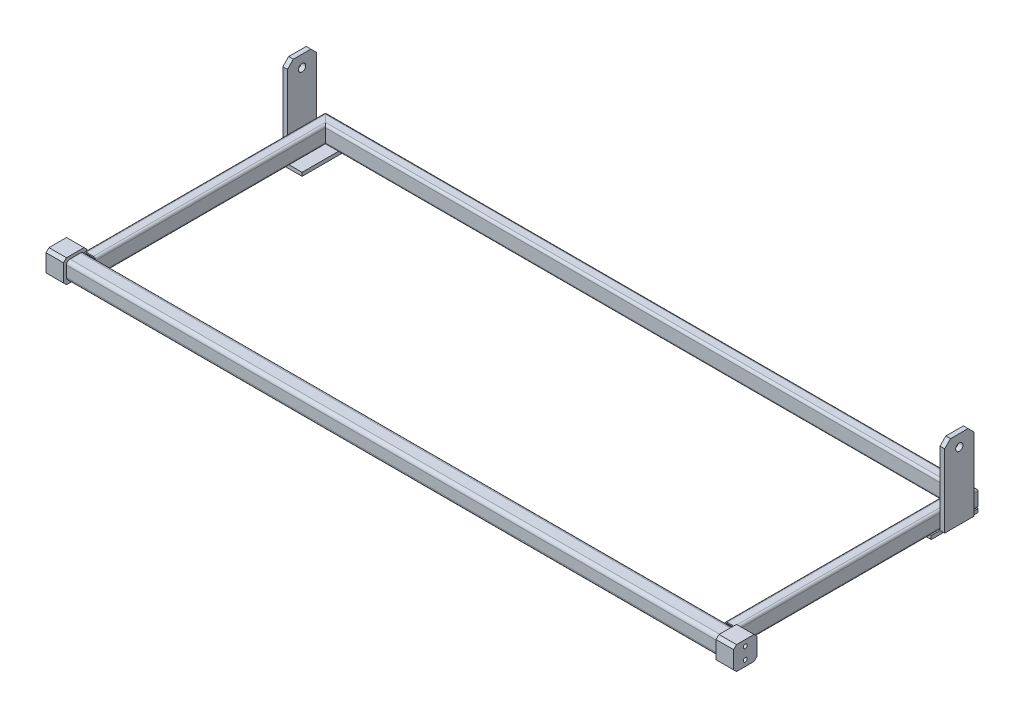
SolidWorks part; units mm, degrees
ref_plane "Front Plane" through (0, 0, 0) normal (0, 0, 1) x (1, 0, 0)
ref_plane "Top Plane" through (0, 0, 0) normal (0, 1, 0) x (1, 0, 0)
ref_plane "Right Plane" through (0, 0, 0) normal (1, 0, 0) x (0, 0, -1)
sketch3d "3DSketch2"
  line L0 (0, 0, 0) -> (1116, 0, 0)
  dimension "D1" = 1116
other "Cold-formed hollow square steel (GB/T 6728-2002) 30×3(1)"
ref_plane "Plane1" through (0, 0, 0) normal (1, 0, 0) x (0, 0, -1)
sketch "Sketch11" plane through (0, 0, 0) normal (1, 0, 0) x (0, 0, -1)
  line L0 (-9, -12) -> (9, -12)
  line L1 (-12, -9) -> (-12, 9)
  line L2 (9, 12) -> (-9, 12)
  line L3 (12, 9) -> (12, -9)
  line L4 (-9, -15) -> (9, -15)
  line L5 (-15, -9) -> (-15, 9)
  line L6 (9, 15) -> (-9, 15)
  line L7 (15, 9) -> (15, -9)
  arc A0 (15, 9) -> (9, 15) centre (9, 9) ccw
  arc A1 (9, -15) -> (15, -9) centre (9, -9) ccw
  arc A2 (-15, -9) -> (-9, -15) centre (-9, -9) ccw
  arc A3 (-9, 15) -> (-15, 9) centre (-9, 9) ccw
  arc A4 (-9, 12) -> (-12, 9) centre (-9, 9) ccw
  arc A5 (12, 9) -> (9, 12) centre (9, 9) ccw
  arc A6 (9, -12) -> (12, -9) centre (9, -9) ccw
  arc A7 (-12, -9) -> (-9, -12) centre (-9, -9) ccw
  point P0 (-15, 0)
  point P1 (15, 0)
  point P2 (0, 15)
  point P3 (0, -15)
  point P4 (0, 0)
  point P5 (-15, -15)
  point P6 (15, -15)
  point P7 (15, 15)
  point P8 (-15, 15)
  point P33 (0, 0)
  dimension "D1" = 6
  dimension "D2" = 30
  dimension "D3" = 3
sketch3d "3DSketch3"
  line L0 (1106, 0, -15) -> (1106, 0, -418)
  line L2 (10, 0, -15) -> (10, 0, -418)
  line L3 (10, 0, -15) -> (1106, 0, -15) construction
  line L4 (10, 0, -418) -> (1106, 0, -418)
  dimension "D1" = 10
  dimension "D2" = 10
  dimension "D3" = 403
other "Cold-formed hollow rectangular steel (GB/T 6728-2002) 30×20×2(1)"
ref_plane "Plane2" through (1106, 0, -15) normal (0, 0, -1) x (1, 0, 0)
sketch "Sketch1" plane through (1106, 0, -15) normal (0, 0, -1) x (1, 0, 0)
  line L0 (-6, -13) -> (6, -13)
  line L1 (-8, -11) -> (-8, 11)
  line L2 (6, 13) -> (-6, 13)
  line L3 (8, 11) -> (8, -11)
  line L4 (-6, -15) -> (6, -15)
  line L5 (-10, -11) -> (-10, 11)
  line L6 (6, 15) -> (-6, 15)
  line L7 (10, 11) -> (10, -11)
  arc A0 (10, 11) -> (6, 15) centre (6, 11) ccw
  arc A1 (6, -15) -> (10, -11) centre (6, -11) ccw
  arc A2 (-10, -11) -> (-6, -15) centre (-6, -11) ccw
  arc A3 (-6, 15) -> (-10, 11) centre (-6, 11) ccw
  arc A4 (-6, 13) -> (-8, 11) centre (-6, 11) ccw
  arc A5 (8, 11) -> (6, 13) centre (6, 11) ccw
  arc A6 (6, -13) -> (8, -11) centre (6, -11) ccw
  arc A7 (-8, -11) -> (-6, -13) centre (-6, -11) ccw
  point P0 (0, 15)
  point P1 (10, 0)
  point P2 (0, -15)
  point P3 (-10, 0)
  point P4 (-10, 15)
  point P5 (10, 15)
  point P6 (10, -15)
  point P7 (-10, -15)
  point P8 (0, 0)
  point P33 (0, 0)
  dimension "D1" = 30
  dimension "D2" = 20
  dimension "D3" = 2
  dimension "D4" = 4
sketch "Sketch4" plane through (0, 0, 0) normal (-1, 0, 0) x (0, 0, 1)
  line L0 (-20, 15) -> (-15, 20)
  line L1 (15, -20) -> (-15, -20)
  line L2 (20, -15) -> (20, 15)
  line L3 (15, 20) -> (-15, 20)
  line L4 (-20, -15) -> (-20, 15)
  line L5 (20, -20) -> (-20, 20) construction
  line L6 (20, 20) -> (-20, -20) construction
  line L7 (20, 15) -> (15, 20)
  line L8 (15, -20) -> (20, -15)
  line L9 (-15, -20) -> (-20, -15)
  point P0 (0, 0)
  dimension "D1" = 40
extrude "Boss-Extrude1" add sketch "Sketch4" along normal blind 30 separate body
sketch "Sketch5" plane through (-30, 0, 0) normal (-1, 0, 0) x (0, 0, 1)
  line L0 (0, 20) -> (0, -20) construction
  line L1 (15, 20) -> (-15, 20) construction
  line L2 (-15, -20) -> (15, -20) construction
  circle A0 centre (0, 10) radius 1.7011
  circle A1 centre (0, -10) radius 1.7011
  dimension "D1" = 3.4021
  dimension "D3" = 20
  dimension "D2" = 10
extrude "Cut-Extrude1" cut sketch "Sketch5" against normal blind 30
hole_wizard "M8 Tapped Hole1" positions "3DSketch4" profile "Sketch6" tap size "M8" standard "GB"
sketch3d "3DSketch4"
  line L0 (0, 10, 0) -> (-30, 10, 0) construction
  line L1 (0, -10, 0) -> (-30, -10, 0) construction
  point P0 (-30, 10, 0)
  point P4 (-30, -10, 0)
sketch "Sketch6" plane through (-30, 10, 0) normal (0, 1, 0) x (0, 0, 1)
  line L0 (0, 0) -> (0, 32.0429)
  line L1 (0, 32.0429) -> (3.4, 30)
  line L2 (3.4, 30) -> (3.4, 0)
  line L5 (3.4, 0) -> (0, 0)
  line L10 (0, 32.0429) -> (-3.4, 30) construction
  line L11 (0, -6.35) -> (0, 107.95) construction
  dimension "螺纹孔钻头直径" = 6.8
  dimension "螺纹孔钻头深度" = 30
  dimension "导头角度" = 118
cosmetic thread "Hole thread1" parameters "D1"=16, "D2"=8
cosmetic thread "Hole thread2" parameters "D1"=16, "D2"=8
ref_plane "Plane3" through (558, 0, 0) normal (-1, 0, 0) x (0, 0, 1)
sketch "Sketch7" plane through (0, -15, 0) normal (0, -1, 0) x (1, 0, 0)
  line L9 (1116, -428) -> (1076, -428)
  line L10 (1116, -428) -> (1116, -348)
  line L11 (1116, -348) -> (1076, -348)
  line L12 (1076, -428) -> (1076, -348)
  line L13 (0, -428) -> (40, -428)
  line L14 (0, -428) -> (0, -348)
  line L15 (0, -348) -> (40, -348)
  line L16 (40, -428) -> (40, -348)
  dimension "D1" = 40
  dimension "D2" = 80
  dimension "D3" = 40
  dimension "D4" = 80
extrude "Boss-Extrude2" add sketch "Sketch7" along normal blind 6 separate body
ref_plane "Plane4" through (0, -11, -428) normal (0, 0, -1) x (-1, 0, 0)
sketch "Sketch9" plane through (0, 0, 0) normal (-1, 0, 0) x (0, 0, 1)
  line L0 (-348, -15) -> (-428, -15) construction
  line L1 (-413, -15) -> (-363, -15)
  line L2 (-413, -15) -> (-413, 110)
  line L3 (-403, 120) -> (-373, 120)
  line L4 (-363, -15) -> (-363, 110)
  line L5 (-428, 102.575) -> (-428, -124.575) construction
  line L6 (-413, 110) -> (-403, 120)
  line L7 (-373, 120) -> (-363, 110)
  line L8 (-388, 120) -> (-388, 26.5616) construction
  circle A0 centre (-388, 100) radius 6.25
  point P1 (-363, 120)
  point P2 (-413, 120)
  dimension "D4" = 20
  dimension "D5" = 12.5
  dimension "D1" = 135
  dimension "D2" = 15
  dimension "D3" = 50
extrude "Boss-Extrude3" add sketch "Sketch9" along normal blind 8 separate body
mirror "Mirror1" about plane through (558, 0, 0) normal (-1, 0, 0) of "Boss-Extrude3", "Boss-Extrude1", "Cut-Extrude1", "M8 Tapped Hole1"
sketch "Sketch10" plane through (0, 0, -428) normal (0, 0, -1) x (-1, 0, 0)
  line L0 (-1116, 0) -> (-932.0936, 0) construction
  line L1 (0, 0) -> (-1116, 0) construction
  line L2 (-1116, 110) -> (-1116, 11) construction
  circle A0 centre (-776, 0) radius 2
  circle A1 centre (-741, 0) radius 2
  circle A2 centre (-706, 0) radius 2
  circle A3 centre (-671, 0) radius 2
  dimension "D1" = 4
  dimension "D2" = 35
  dimension "D3" = 35
  dimension "D4" = 35
  dimension "D5" = 340
extrude "Cut-Extrude2" cut sketch "Sketch10" against normal blind 8
hole_wizard "M6 Tapped Hole1" positions "3DSketch5" profile "草图11" tap size "M6" standard "GB"
sketch3d "3DSketch5"
  line L0 (671, 0, -426) -> (671, 0, -428) construction
  line L1 (706, 0, -426) -> (706, 0, -428) construction
  line L2 (741, 0, -426) -> (741, 0, -428) construction
  line L3 (776, 0, -426) -> (776, 0, -428) construction
  point P0 (671, 0, -428)
  point P4 (706, 0, -428)
  point P8 (741, 0, -428)
  point P12 (776, 0, -428)
sketch "草图11" plane through (671, 0, -428) normal (1, 0, 0) x (0, 1, 0)
  line L0 (0, 0) -> (0, 18.5022)
  line L1 (0, 18.5022) -> (2.5, 17)
  line L2 (2.5, 17) -> (2.5, 0)
  line L5 (2.5, 0) -> (0, 0)
  line L10 (0, 18.5022) -> (-2.5, 17) construction
  line L11 (0, -6.35) -> (0, 107.95) construction
  dimension "螺纹孔钻头直径" = 5
  dimension "螺纹孔钻头深度" = 17
  dimension "导头角度" = 118
cosmetic thread "Hole thread3" parameters "D1"=2, "D2"=6
cosmetic thread "Hole thread4" parameters "D1"=2, "D2"=6
cosmetic thread "Hole thread5" parameters "D1"=2, "D2"=6
cosmetic thread "Hole thread6" parameters "D1"=2, "D2"=6
